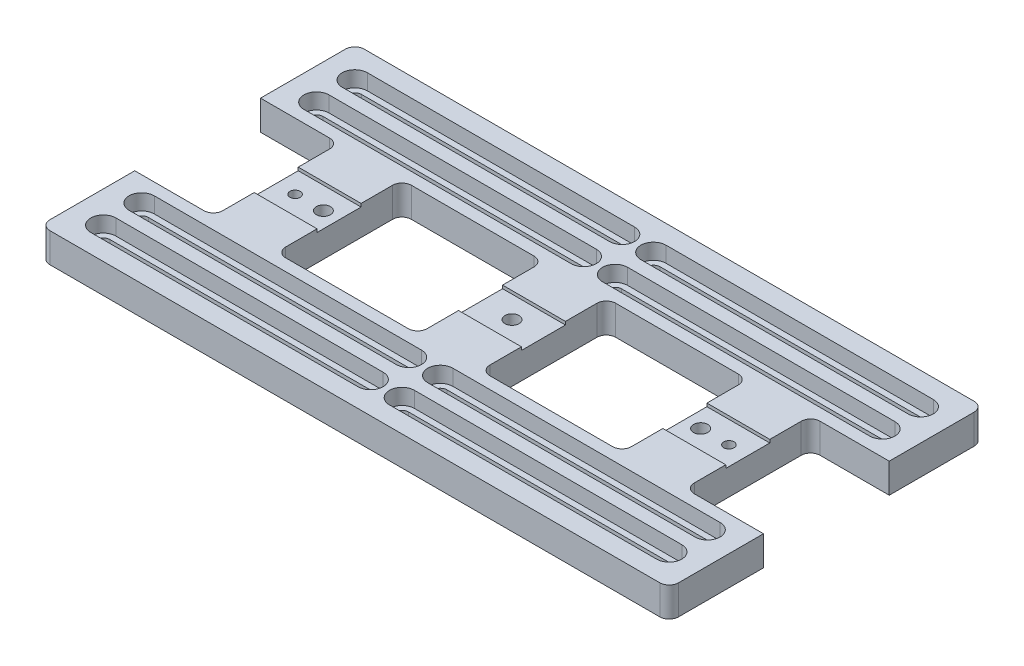
from build123d import *

# Parameters (mm, degrees)
SKETCH1_W                                            = 200
SKETCH1_H                                            = 100
BOSS_EXTRUDE1_DEPTH                                  = 4.7
FILLET1_R                                            = 3
SKETCH2_W                                            = 50
SKETCH2_H                                            = 40
CUT_EXTRUDE1_DEPTH                                   = 113.197860942
SKETCH3_W                                            = 45
SKETCH3_H                                            = 40
CUT_EXTRUDE2_DEPTH                                   = 113.197860942
FILLET2_R                                            = 3
FILLET3_R                                            = 3
FILLET3_OF_MIRROR2_R                                 = 3
CUT_EXTRUDE3_DEPTH                                   = 5
CUT_EXTRUDE4_DEPTH                                   = 112.915146428
MIRROR3_AT_THE_SECOND_PLANE_COPY_1_DEPTH             = 5
MIRROR3_AT_THE_SECOND_PLANE_COPY_2_DEPTH             = 112.915146428
SKETCH6_W                                            = 150
SKETCH6_H                                            = 14
CUT_EXTRUDE5_DEPTH                                   = 1
M4_TAPPED_HOLE1_D                                    = 3.3
M4_TAPPED_HOLE1_DEPTH                                = 11.5
M4_TAPPED_HOLE1_TIP                                  = 0.991420021
CBORE_FOR_M4_HEXAGON_SOCKET_HEAD_CAP_SCR_D           = 4.5
CBORE_FOR_M4_HEXAGON_SOCKET_HEAD_CAP_SCR_DEPTH       = 11.5
CBORE_FOR_M4_HEXAGON_SOCKET_HEAD_CAP_SCR_CBORE_D     = 8
CBORE_FOR_M4_HEXAGON_SOCKET_HEAD_CAP_SCR_CBORE_DEPTH = 4.6
CBORE_FOR_M4_HEXAGON_SOCKET_HEAD_CAP_SCR_TIP         = 1.351936393


with BuildPart() as part:
    # Sketch1 → Boss-Extrude1 (new, symmetric)
    with BuildSketch(Plane(origin=(0, 0, 0), x_dir=(1, 0, 0), z_dir=(0, 1, 0))):
        Rectangle(SKETCH1_W, SKETCH1_H)
    extrude(amount=BOSS_EXTRUDE1_DEPTH, both=True)

    # Fillet1
    fillet1_edges = [part.edges().sort_by_distance(p)[0] for p in [
        (-100, 0, -50),
        (100, 0, -50),
        (100, 0, 50),
        (-100, 0, 50),
    ]]
    fillet(fillet1_edges, radius=FILLET1_R)

    # Sketch2 → Cut-Extrude1 (cut, through all)
    with BuildSketch(Plane(origin=(0, 4.7, 0), x_dir=(1, 0, 0), z_dir=(0, 1, 0))):
        with Locations((100, 0)):
            Rectangle(SKETCH2_W, SKETCH2_H)
    cut_extrude1 = extrude(amount=-CUT_EXTRUDE1_DEPTH, mode=Mode.SUBTRACT)

    # Mirror1: Cut-Extrude1 across plane
    add(cut_extrude1.mirror(Plane(origin=(0, 0, 0), x_dir=(0, 0, 1), z_dir=(1, 0, 0))), mode=Mode.SUBTRACT)

    # Sketch3 → Cut-Extrude2 (cut, through all)
    with BuildSketch(Plane(origin=(0, 4.7, 0), x_dir=(1, 0, 0), z_dir=(0, 1, 0))):
        with Locations((-32.5, 0)):
            Rectangle(SKETCH3_W, SKETCH3_H)
    cut_extrude2 = extrude(amount=-CUT_EXTRUDE2_DEPTH, mode=Mode.SUBTRACT)

    # Fillet2
    fillet2_edges = [part.edges().sort_by_distance(p)[0] for p in [
        (75, 0, -20),
        (75, 0, 20),
        (-75, 0, 20),
        (-75, 0, -20),
    ]]
    fillet(fillet2_edges, radius=FILLET2_R)

    # Fillet3
    fillet3_edges = [part.edges().sort_by_distance(p)[0] for p in [
        (-55, 0, 20),
        (-55, 0, -20),
        (-10, 0, -20),
        (-10, 0, 20),
    ]]
    fillet(fillet3_edges, radius=FILLET3_R)

    # Mirror2: Cut-Extrude2 across plane
    add(cut_extrude2.mirror(Plane(origin=(0, 0, 0), x_dir=(0, 0, 1), z_dir=(1, 0, 0))), mode=Mode.SUBTRACT)

    # Fillet3 of Mirror2
    fillet3_of_mirror2_edges = [part.edges().sort_by_distance(p)[0] for p in [
        (55, 0, 20),
        (55, 0, -20),
        (10, 0, -20),
        (10, 0, 20),
    ]]
    fillet(fillet3_of_mirror2_edges, radius=FILLET3_OF_MIRROR2_R)

    # Sketch4 → Cut-Extrude3 (cut)
    with BuildSketch(Plane(origin=(0, 4.7, 0), x_dir=(1, 0, 0), z_dir=(0, 1, 0))):
        with BuildLine():
            Line((-90, -36), (-5, -36))
            ThreePointArc((-5, -36), (-1, -40), (-5, -44))
            Line((-5, -44), (-90, -44))
            ThreePointArc((-90, -44), (-94, -40), (-90, -36))
        make_face()
        with BuildLine():
            Line((-90, -31.8), (-5, -31.8))
            ThreePointArc((-5, -31.8), (-1, -27.8), (-5, -23.8))
            Line((-5, -23.8), (-90, -23.8))
            ThreePointArc((-90, -23.8), (-94, -27.8), (-90, -31.8))
        make_face()
    cut_extrude3 = extrude(amount=-CUT_EXTRUDE3_DEPTH, mode=Mode.SUBTRACT)

    # Sketch5 → Cut-Extrude4 (cut, through all)
    with BuildSketch(Plane(origin=(0, -0.3, 0), x_dir=(1, 0, 0), z_dir=(0, 1, 0))):
        with BuildLine():
            Line((-90, -25.7), (-5, -25.7))
            ThreePointArc((-5, -25.7), (-2.9, -27.8), (-5, -29.9))
            Line((-5, -29.9), (-90, -29.9))
            ThreePointArc((-90, -29.9), (-92.1, -27.8), (-90, -25.7))
        make_face()
        with BuildLine():
            Line((-90, -37.9), (-5, -37.9))
            ThreePointArc((-5, -37.9), (-2.9, -40), (-5, -42.1))
            Line((-5, -42.1), (-90, -42.1))
            ThreePointArc((-90, -42.1), (-92.1, -40), (-90, -37.9))
        make_face()
    cut_extrude4 = extrude(amount=-CUT_EXTRUDE4_DEPTH, mode=Mode.SUBTRACT)

    # Mirror3: Cut-Extrude3, Cut-Extrude4 across plane
    add(cut_extrude3.mirror(Plane(origin=(0, 0, 0), x_dir=(0, 0, 1), z_dir=(1, 0, 0))), mode=Mode.SUBTRACT)
    add(cut_extrude4.mirror(Plane(origin=(0, 0, 0), x_dir=(0, 0, 1), z_dir=(1, 0, 0))), mode=Mode.SUBTRACT)

    # Mirror3 at the second plane: Cut-Extrude3, Cut-Extrude4 across plane
    add(cut_extrude3.mirror(Plane.XY), mode=Mode.SUBTRACT)
    add(cut_extrude4.mirror(Plane.XY), mode=Mode.SUBTRACT)

    # Mirror3 at the second plane copy 1 sketc → Mirror3 at the second plane copy 1 (cut)
    with BuildSketch(Plane(origin=(0, 4.7, 0), x_dir=(-1, 0, 0), z_dir=(0, 1, 0))):
        with BuildLine():
            Line((-90, -36), (-5, -36))
            ThreePointArc((-5, -36), (-1, -40), (-5, -44))
            Line((-5, -44), (-90, -44))
            ThreePointArc((-90, -44), (-94, -40), (-90, -36))
        make_face()
        with BuildLine():
            Line((-90, -31.8), (-5, -31.8))
            ThreePointArc((-5, -31.8), (-1, -27.8), (-5, -23.8))
            Line((-5, -23.8), (-90, -23.8))
            ThreePointArc((-90, -23.8), (-94, -27.8), (-90, -31.8))
        make_face()
    extrude(amount=-MIRROR3_AT_THE_SECOND_PLANE_COPY_1_DEPTH, mode=Mode.SUBTRACT)

    # Mirror3 at the second plane copy 2 sketc → Mirror3 at the second plane copy 2 (cut, through all)
    with BuildSketch(Plane(origin=(0, -0.3, 0), x_dir=(-1, 0, 0), z_dir=(0, 1, 0))):
        with BuildLine():
            Line((-90, -25.7), (-5, -25.7))
            ThreePointArc((-5, -25.7), (-2.9, -27.8), (-5, -29.9))
            Line((-5, -29.9), (-90, -29.9))
            ThreePointArc((-90, -29.9), (-92.1, -27.8), (-90, -25.7))
        make_face()
        with BuildLine():
            Line((-90, -37.9), (-5, -37.9))
            ThreePointArc((-5, -37.9), (-2.9, -40), (-5, -42.1))
            Line((-5, -42.1), (-90, -42.1))
            ThreePointArc((-90, -42.1), (-92.1, -40), (-90, -37.9))
        make_face()
    extrude(amount=-MIRROR3_AT_THE_SECOND_PLANE_COPY_2_DEPTH, mode=Mode.SUBTRACT)

    # Sketch6 → Cut-Extrude5 (cut)
    with BuildSketch(Plane(origin=(0, 4.7, 0), x_dir=(1, 0, 0), z_dir=(0, 1, 0))):
        Rectangle(SKETCH6_W, SKETCH6_H)
    extrude(amount=-CUT_EXTRUDE5_DEPTH, mode=Mode.SUBTRACT)

    # M4 Tapped Hole1
    with Locations(Plane(origin=(0, -4.7, 0), x_dir=(-1, 0, 0), z_dir=(0, -1, 0))):
        with Locations((-69, 0), (69, 0)):
            Hole(M4_TAPPED_HOLE1_D / 2, depth=M4_TAPPED_HOLE1_DEPTH)
            with Locations((0, 0, -(M4_TAPPED_HOLE1_DEPTH + M4_TAPPED_HOLE1_TIP / 2))):  # 118° drill point
                Cone(0, M4_TAPPED_HOLE1_D / 2, M4_TAPPED_HOLE1_TIP, mode=Mode.SUBTRACT)

    # CBORE for M4 Hexagon socket head cap screws1
    with Locations(Plane(origin=(0, -4.7, 0), x_dir=(-1, 0, 0), z_dir=(0, -1, 0))):
        with Locations((-60, 0), (0, 0), (60, 0)):
            CounterBoreHole(CBORE_FOR_M4_HEXAGON_SOCKET_HEAD_CAP_SCR_D / 2, CBORE_FOR_M4_HEXAGON_SOCKET_HEAD_CAP_SCR_CBORE_D / 2, CBORE_FOR_M4_HEXAGON_SOCKET_HEAD_CAP_SCR_CBORE_DEPTH, depth=CBORE_FOR_M4_HEXAGON_SOCKET_HEAD_CAP_SCR_DEPTH)
            with Locations((0, 0, -(CBORE_FOR_M4_HEXAGON_SOCKET_HEAD_CAP_SCR_DEPTH + CBORE_FOR_M4_HEXAGON_SOCKET_HEAD_CAP_SCR_TIP / 2))):  # 118° drill point
                Cone(0, CBORE_FOR_M4_HEXAGON_SOCKET_HEAD_CAP_SCR_D / 2, CBORE_FOR_M4_HEXAGON_SOCKET_HEAD_CAP_SCR_TIP, mode=Mode.SUBTRACT)


solid = part.part
